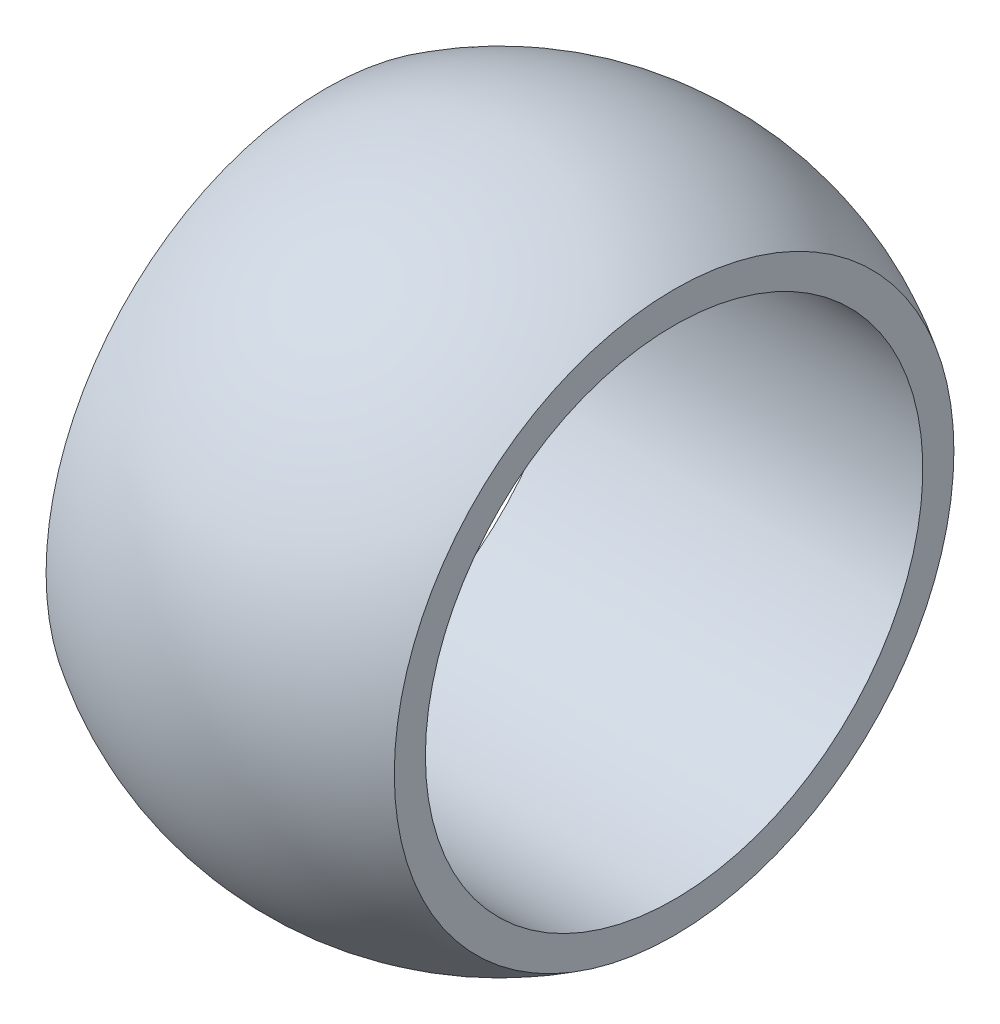
from build123d import *


with BuildPart() as part:
    # 草图1 → 旋转1 (revolve)
    with BuildSketch(Plane.XY, mode=Mode.PRIVATE) as revolve_1_sk:
        with BuildLine():
            Line((-14, 22.5), (-14, 20))
            Line((-14, 20), (14, 20))
            Line((14, 20), (14, 22.5))
            ThreePointArc((14, 22.5), (0, 26.5), (-14, 22.5))
        make_face()
    revolve(revolve_1_sk.sketch.rotate(Axis((-51.72060984, 0, 0), (1, 0, 0)), 90), axis=Axis((-51.72060984, 0, 0), (1, 0, 0)))


solid = part.part
